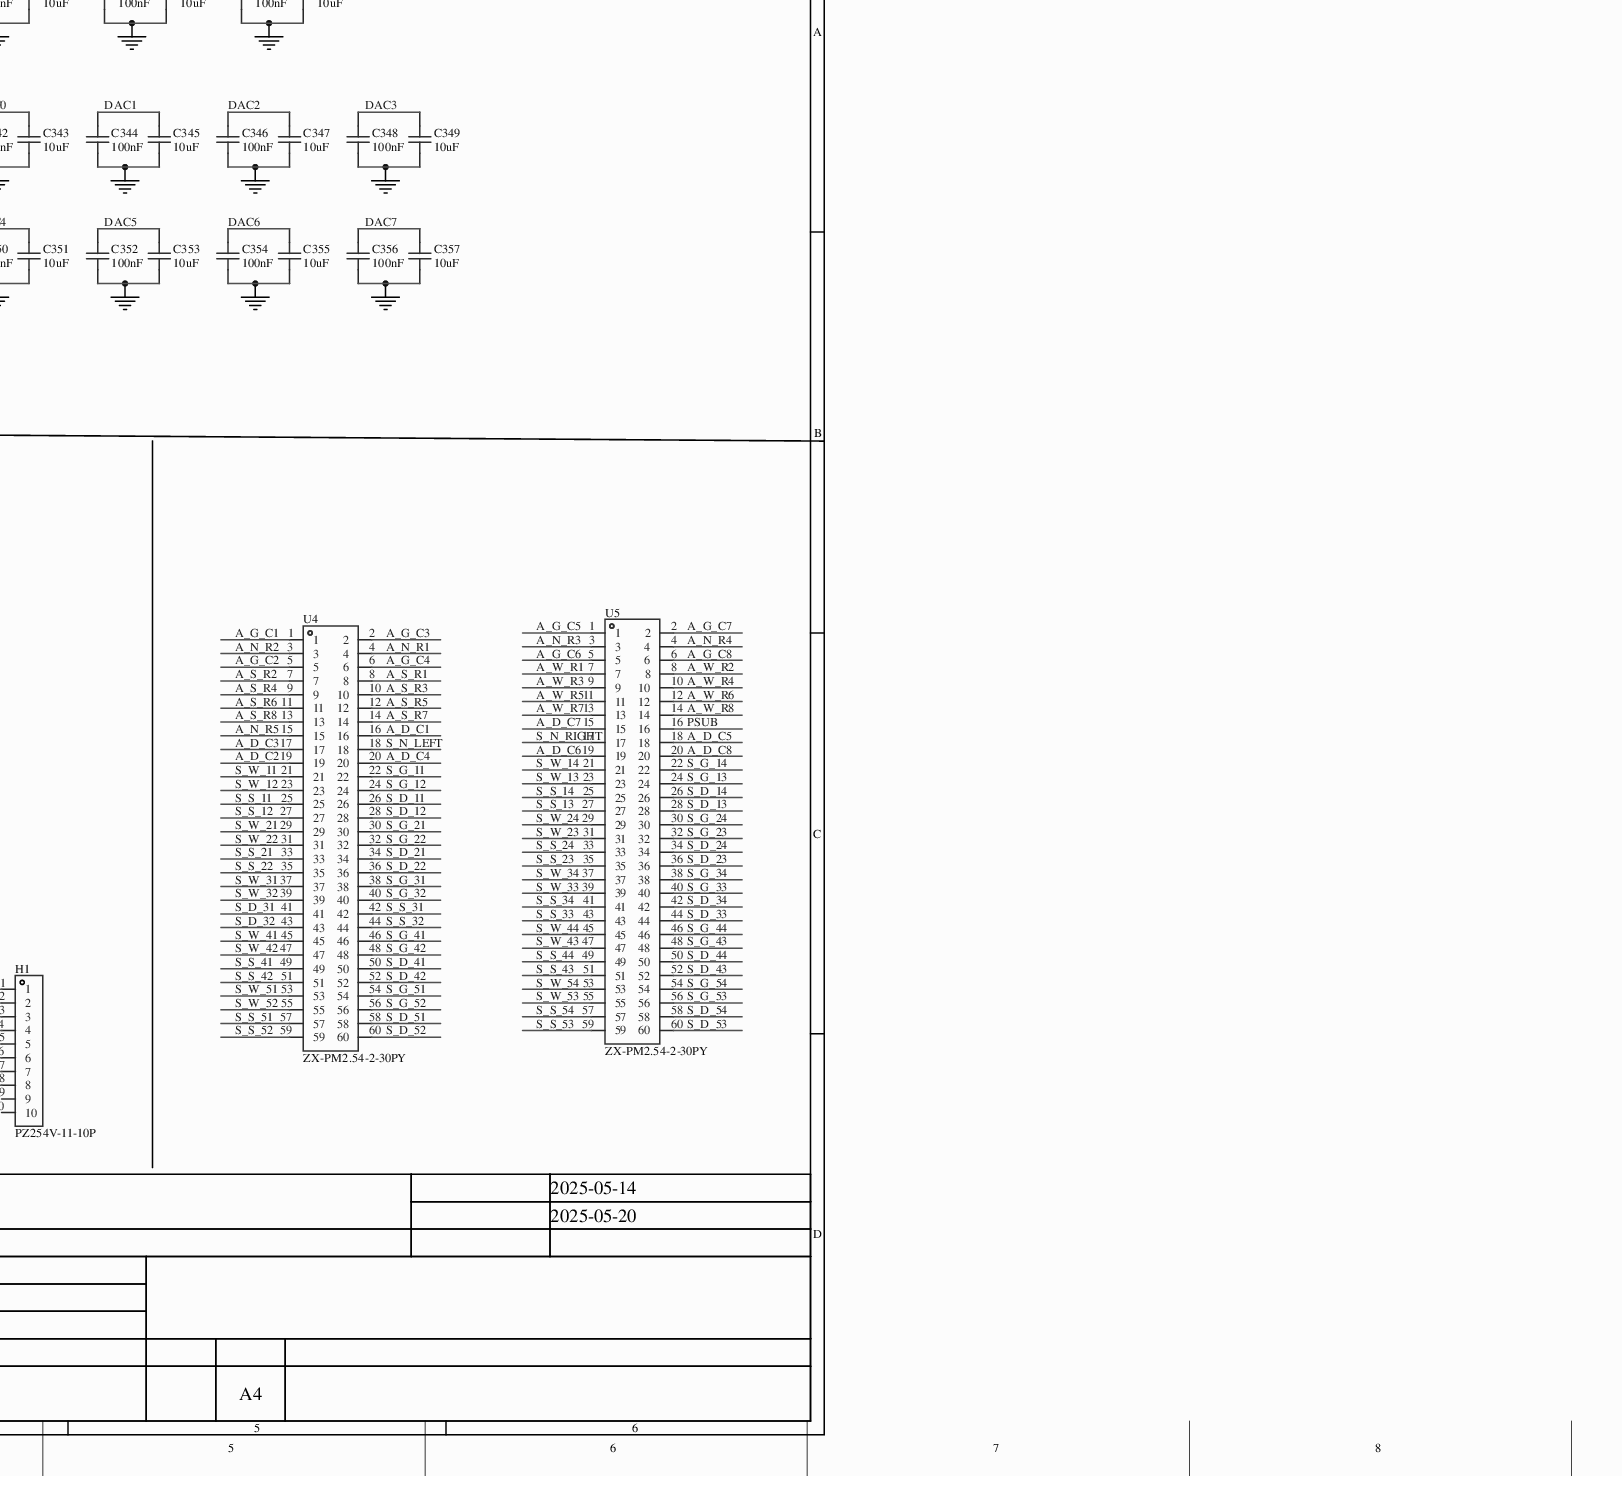
[diagram p0: MISC82799-2.schdoc, bottom column 2 of 4]
# Altium project MISC82799-9.PrjPCB (part 2 of 3)
## Sheet MISC82799-2.schdoc (continued)
### Library data of the parts (continued)
C330 = GRM21BR61H106KE43L: Add into BOM: yes; Voltage Rated: 50V; Temperature Coefficient: X5R; Symbol: 10uF; Device: GRM21BR61H106KE43L; Supplier Part: C440198; Manufacturer Part: GRM21BR61H106KE43L; Supplier Footprint: 0805; JLCPCB Part Class: Basic Part; Datasheet: https://example.com/upload/public/pdf/source/20230811/95AAE0C9AF55EDC31B7A4D8B733F534E.pdf; Supplier: LCSC; Convert to PCB: yes; Value: 10uF
C358 C359 = CL10A225KB8NNNC: Add into BOM: yes; Voltage Rated: 50V; Temperature Coefficient: X5R; Symbol: CL10A225KB8NNNC; Device: CL10A225KB8NNNC; Supplier Part: C913904; Manufacturer Part: CL10A225KB8NNNC; Supplier Footprint: 0603; Datasheet: https://example.com/upload/public/pdf/source/20160218/1457707763339.pdf; Supplier: LCSC; Convert to PCB: yes; Value: 2.2uF; Origin Footprint: C0603
C361-C363 = CL10A105KB8NNNC: Add into BOM: yes; Voltage Rated: 50V; Temperature Coefficient: X5R; Symbol: CL10A105KB8NNNC; Device: CL10A105KB8NNNC; Supplier Part: C15849; Manufacturer Part: CL10A105KB8NNNC; Supplier Footprint: 0603; Datasheet: https://example.com/upload/public/pdf/source/20160218/1457707763339.pdf; Supplier: LCSC; Convert to PCB: yes; Value: 1uF; Origin Footprint: C0603
D1 = VS-10BQ015HM3/5BT: Add into BOM: yes; Forward Voltage (Vf@If): 210mV@1A; Reverse Voltage (Vr): 15V; Rectified Current: 1A; Reverse Leakage Current (Ir): 500uA@15V; Symbol: VS-10BQ015HM3/5BT; Device: VS-10BQ015HM3/5BT; Supplier Part: C413465; Manufacturer Part: VS-10BQ015HM3/5BT; Supplier Footprint: DO-214AA(SMB); JLCPCB Part Class: Extended Part; Datasheet: https://example.com/upload/public/pdf/source/20190819/C413465_3D2B1A8C7366D4425AB887DF85498F89.pdf; Supplier: LCSC; Convert to PCB: yes
FPGAJ2 FPGAJ4 FPGAJ10 = 2.54-2*20: Add into BOM: yes; Holes Structure: 2x20P; Pitch: 2.54mm; Number of Holes: 40P; Current Rating (Max): 2.5A; Symbol: 2.54-2*20; Device: 2.54-2*20; Supplier Part: C2977589; Manufacturer Part: 2.54-2*20; JLCPCB Part Class: Extended Part; Datasheet: https://example.com/upload/public/pdf/source/20220328/834E302BE3C038BBC5C70F5E02589B1E.pdf; Supplier: LCSC; Convert to PCB: yes; Row Spacing: 2.54mm; Voltage Rating (Max): -; Insulation Height: 8.5mm
H1 = PZ254V-11-10P: Add into BOM: yes; Pin Structure: 1x10P; Pitch: 2.54mm; Symbol: PZ254V-11-10P; Device: PZ254V-11-10P; Supplier Part: C492409; Manufacturer Part: PZ254V-11-10P; JLCPCB Part Class: Extended Part; Datasheet: https://example.com/upload/public/pdf/source/20200309/C492409_129C9431BDD62EBBBD0A643B6AAB9FBD.pdf; Supplier: LCSC; Convert to PCB: yes; Row Spacing: -; Number of Pins: 10P; Current Rating: -; Voltage Rating (Max): -; Length of Mating Pin: 6mm; Insulation Height: 2.5mm; Length of End Connection Pin: 3mm; Contact Plating: -
H2 = PZ254-2-20-W-8.5_C2895000: Add into BOM: yes; Pin Structure: 2x20P; Pitch: 2.54mm; Current Rating (Max): 3A; Symbol: PZ254-2-20-W-8.5; Device: PZ254-2-20-W-8.5_C2895000; Supplier Part: C2895000; Manufacturer Part: PZ254-2-20-W-8.5; JLCPCB Part Class: Extended Part; Datasheet: https://example.com/upload/public/pdf/source/20230609/1B60364E488FD8696AA7206A46578DEA.pdf; Supplier: LCSC; Convert to PCB: yes; Row Spacing: 2.54mm; Number of Pins: 40P; Voltage Rating (Max): -; Length of Mating Pin: 6mm; Insulation Height: 2.5mm; Length of End Connection Pin: -; Contact Material: -
H3 = PZ254V-12-16P: Add into BOM: yes; Pin Structure: 2x8P; Pitch: 2.54mm; Symbol: PZ254V-12-16P; Device: PZ254V-12-16P; Supplier Part: C492425; Manufacturer Part: PZ254V-12-16P; JLCPCB Part Class: Extended Part; Datasheet: https://example.com/upload/public/pdf/source/20200309/C492425_0A00EE06259AD0A0AB9C88167BB69964.pdf; Supplier: LCSC; Convert to PCB: yes; Row Spacing: 2.54mm; Number of Pins: 16P; Current Rating: -; Voltage Rating (Max): -; Length of Mating Pin: 6mm; Insulation Height: 2.5mm; Length of End Connection Pin: 3mm; Contact Plating: -
H7 H9 = PZ254V-11-03P: Add into BOM: yes; Pin Structure: 1x3P; Pitch: 2.54mm; Current Rating: 3A; Voltage Rating (Max): 250V; Symbol: PZ254V-11-03P; Device: PZ254V-11-03P; Supplier Part: C2937625; Manufacturer Part: PZ254V-11-03P; Datasheet: https://example.com/upload/public/pdf/source/20200309/C492402_8335C3D49C4E4C618838D59BB1D024C1.pdf; Supplier: LCSC; Convert to PCB: yes; Row Spacing: -; Number of Pins: 3P; Length of Mating Pin: 6mm; Insulation Height: 2.5mm; Length of End Connection Pin: 3mm; Origin Footprint: HDR-TH_3P-P2.54-V-M
H8 = PZ254V-11-05P: Add into BOM: yes; Pin Structure: 1x5P; Pitch: 2.54mm; Symbol: PZ254V-11-05P; Device: PZ254V-11-05P; Supplier Part: C492404; Manufacturer Part: PZ254V-11-05P; Datasheet: https://example.com/upload/public/pdf/source/20200309/C492404_E51533260F8710EFF5D4617281164C1D.pdf; Supplier: LCSC; Convert to PCB: yes; Row Spacing: -; Number of Pins: 5P; Current Rating: -; Voltage Rating (Max): -; Length of Mating Pin: 6mm; Insulation Height: 2.5mm; Length of End Connection Pin: 3mm; Contact Plating: -; Origin Footprint: HDR-TH_5P-P2.54-V-M
L3 = PCAQ7060MW-301: Add into BOM: yes; Number of Lines: 2; Voltage Withstand: 125V; Current Rating: 5A; Symbol: PCAQ7060MW-301; Device: PCAQ7060MW-301; Supplier Part: C2916896; Manufacturer Part: PCAQ7060MW-301; Supplier Footprint: SMD,7x6x3.8mm; Datasheet: https://example.com/upload/public/pdf/source/20220923/2764902BE544E236930A8CC0DC83284B.pdf; Supplier: LCSC; Convert to PCB: yes; Inductance @ Frequency: -; Voltage Rating - DC: 125V; Voltage Rating (AC): -; Origin Footprint: FILTER-SMD_4P-L7.0-W6.0-BL
LED1 = NCD0805G1: Add into BOM: yes; Forward Voltage (VF): 2.5V~3.6V; Power Dissipation: 72mW; Forward Current: 5mA; Dominant Wavelength: 525nm~537.5nm; Luminous Intensity: 180mcd~400mcd; Symbol: NCD0805G1; Device: NCD0805G1; LCSC Part Name: NCD0805G1; Supplier Part: C84260; Manufacturer Part: NCD0805G1; Supplier Footprint: 0805; JLCPCB Part Class: Extended Part; Datasheet: https://example.com/upload/public/pdf/source/20200820/C84260_AFC7BF57C6FBA034D182BB8D10A67EFE.pdf; Supplier: LCSC; Convert to PCB: yes
R25 = 0603WAF1004T5E: Add into BOM: yes; Power(Watts): 100mW; Overload Voltage (Max): 75V; Symbol: 0603WAF1004T5E; Device: 0603WAF1004T5E; Supplier Part: C22935; Manufacturer Part: 0603WAF1004T5E; Supplier Footprint: 0603; JLCPCB Part Class: Basic Part; Datasheet: https://example.com/upload/public/pdf/source/20200306/C422600_1E6D84923E4A46A82E41ADD87F860B5C.pdf; Supplier: LCSC; Convert to PCB: yes
R27 = RT0603BRD07681RL: Add into BOM: yes; Power(Watts): 100mW; Overload Voltage (Max): 75V; Symbol: RT0603BRD07681RL; Device: RT0603BRD07681RL; Supplier Part: C705792; Manufacturer Part: RT0603BRD07681RL; Supplier Footprint: 0603; JLCPCB Part Class: Extended Part; Datasheet: https://example.com/upload/public/pdf/source/20200720/C705792_EDF314EE001EB4AE666F730223633204.pdf; Supplier: LCSC; Convert to PCB: yes
R28 = 0603WAF1001T5E: Add into BOM: yes; Power(Watts): 100mW; Overload Voltage (Max): 75V; Symbol: 0603WAF1001T5E; Device: 0603WAF1001T5E; Supplier Part: C21190; Manufacturer Part: 0603WAF1001T5E; Supplier Footprint: 0603; JLCPCB Part Class: Basic Part; Datasheet: https://example.com/upload/public/pdf/source/20200306/C422600_1E6D84923E4A46A82E41ADD87F860B5C.pdf; Supplier: LCSC; Convert to PCB: yes
R165 = 0603WAF4533T5E: Add into BOM: yes; Power(Watts): 100mW; Overload Voltage (Max): 75V; Symbol: 0603WAF4533T5E; Device: 0603WAF4533T5E; Supplier Part: C25818; Manufacturer Part: 0603WAF4533T5E; Supplier Footprint: 0603; JLCPCB Part Class: Extended Part; Datasheet: https://example.com/upload/public/pdf/source/20200306/C422600_1E6D84923E4A46A82E41ADD87F860B5C.pdf; Supplier: LCSC; Convert to PCB: yes
R166 = AR03BTC5002A: Add into BOM: yes; Power(Watts): 62.5mW; Symbol: AR03BTC5002A; Device: AR03BTC5002A; Supplier Part: C304067; Manufacturer Part: AR03BTC5002A; Supplier Footprint: 0603; JLCPCB Part Class: Extended Part; Datasheet: https://example.com/upload/public/pdf/source/20180929/C304149_5A5914DE4BA6462262A23A17FA3D8526.pdf; Supplier: LCSC; Convert to PCB: yes
R167 = 0603WAF2490T5E: Add into BOM: yes; Power(Watts): 100mW; Overload Voltage (Max): 75V; Symbol: 0603WAF2490T5E; Device: 0603WAF2490T5E; Supplier Part: C22919; Manufacturer Part: 0603WAF2490T5E; Supplier Footprint: 0603; JLCPCB Part Class: Extended Part; Datasheet: https://example.com/upload/public/pdf/source/20200306/C422600_1E6D84923E4A46A82E41ADD87F860B5C.pdf; Supplier: LCSC; Convert to PCB: yes
R168 = 0603WAF2003T5E: Add into BOM: yes; Power(Watts): 100mW; Overload Voltage (Max): 75V; Symbol: 0603WAF2003T5E; Device: 0603WAF2003T5E; Supplier Part: C25811; Manufacturer Part: 0603WAF2003T5E; Supplier Footprint: 0603; JLCPCB Part Class: Basic Part; Datasheet: https://example.com/upload/public/pdf/source/20200306/C422600_1E6D84923E4A46A82E41ADD87F860B5C.pdf; Supplier: LCSC; Convert to PCB: yes
R169 = ERJ3RED3573V: Add into BOM: yes; Power(Watts): 100mW; Voltage-Supply(Max): 100V; Symbol: ERJ3RED3573V; Device: ERJ3RED3573V; Supplier Part: C278649; Manufacturer Part: ERJ3RED3573V; Supplier Footprint: 0603; Datasheet: https://example.com/upload/public/pdf/source/20181114/C278649_3EAAB526D833AC096AA76B5DF119202B.pdf; Supplier: LCSC; Convert to PCB: yes; Origin Footprint: R0603
R170 = 0603WAF7502T5E: Add into BOM: yes; Power(Watts): 100mW; Overload Voltage (Max): 75V; Symbol: 0603WAF7502T5E; Device: 0603WAF7502T5E; Supplier Part: C23242; Manufacturer Part: 0603WAF7502T5E; Supplier Footprint: 0603; Datasheet: https://example.com/upload/public/pdf/source/20200306/C422600_1E6D84923E4A46A82E41ADD87F860B5C.pdf; Supplier: LCSC; Convert to PCB: yes; Origin Footprint: R0603
SW1 = K3-1204D: Add into BOM: yes; Switch Length: 10mm; Switch Width: 2.5mm; Switch Height: 6mm; Current Rating (AC): 5A; Voltage Rating (AC): 120V; Symbol: K3-1204D; Device: K3-1204D; Supplier Part: C145861; Manufacturer Part: K3-1204D; JLCPCB Part Class: Extended Part; Datasheet: https://example.com/upload/public/pdf/source/20210810/A7BCE8A3AE6875067403B729968221B7.pdf; Supplier: LCSC; Convert to PCB: yes; Actuator Style: -; Voltage Rating (DC): -
TP13 = 5V: Add into BOM: yes; Symbol: 5V; Device: 5V; Convert to PCB: yes; Origin Footprint: Test-Point-0.5mm; Design Item ID: Test-Point
TP14 = 3P3V: Add into BOM: yes; Symbol: 3P3V; Device: 3P3V; Convert to PCB: yes; Origin Footprint: Test-Point-0.5mm; Design Item ID: Test-Point
U4 U5 = ZX-PM2.54-2-30PY: Add into BOM: yes; Holes Structure: 2x30P; Pitch: 2.54mm; Number of Holes: 60P; Voltage Rating (Max): 1kV; Symbol: ZX-PM2.54-2-30PY; Device: ZX-PM2.54-2-30PY; Supplier Part: C7499356; Manufacturer Part: ZX-PM2.54-2-30PY; JLCPCB Part Class: Extended Part; Datasheet: https://example.com/upload/public/pdf/source/20231122/23E1107B34356833C267F6B6E856DE02.pdf; Supplier: LCSC; Convert to PCB: yes; Row Spacing: 2.54mm; Current Rating (Max): -; Insulation Height: 8.5mm; Contact Material: -
U39 = HX DC007B-2.5: Add into BOM: yes; Inside Contact Diameter: 2.5mm; Outside Contact Diameter: 6.4mm; Current Rating (Max): 7A; Voltage Rating (Max): 20V; Symbol: HX DC007B-2.5; Device: HX DC007B-2.5; Supplier Part: C19189083; Manufacturer Part: HX DC007B-2.5; JLCPCB Part Class: Extended Part; Datasheet: https://example.com/upload/public/pdf/source/20231103/814B3421283469BAAEFFF9B7A53EC0CB.pdf; Supplier: LCSC; Convert to PCB: yes
U40 = SMAJ12CA: Manufacturer: KUU; Add into BOM: yes; Reverse Stand-Off Voltage (Vrwm): 12V; Maximum Clamping Voltage: 19.9V; Peak Pulse Current (Ipp)@10/1000us: 20.1A; Peak Pulse Power Dissipation (Ppp)@10/1000us: 400W; Breakdown Voltage: 13.3V; Reverse Leakage Current (Ir): 1uA; Symbol: SMAJ12CA; Device: SMAJ12CA; Supplier Part: C2985628; Manufacturer Part: SMAJ12CA; Supplier Footprint: SMA; Datasheet: https://example.com/upload/public/pdf/source/20211202/BA5FA378886C9E49EA844EF3397415D6.pdf; Supplier: LCSC; Convert to PCB: yes; Type: TVS; Origin Footprint: SMA_L4.3-W2.7-LS5.1-BI; Design Item ID: SMAJ12CA
U41 = TPS259472ARPWR: Add into BOM: yes; Voltage Rating: 2.7V~23V; Symbol: TPS259472ARPWR; Device: TPS259472ARPWR; LCSC Part Name: TPS259472ARPWR; Supplier Part: C3662789; Manufacturer Part: TPS259472ARPWR; Supplier Footprint: VQFN-10-HR(2x2); JLCPCB Part Class: Extended Part; Supplier: LCSC; Convert to PCB: yes
U42 U43 = CL21A226KOQNNNE: Add into BOM: yes; Voltage Rated: 16V; Temperature Coefficient: X5R; Symbol: 22uF; Device: CL21A226KOQNNNE; Supplier Part: C296720; Manufacturer Part: CL21A226KOQNNNE; Supplier Footprint: 0805; JLCPCB Part Class: Extended Part; Datasheet: https://example.com/upload/public/pdf/source/20160218/1457707763339.pdf; Supplier: LCSC; Convert to PCB: yes; Value: 22uF
U91 = LT3045IDD#PBF: Add into BOM: yes; Maximum Input Voltage: 20V; Output Voltage: 0V~15V; Output Current: 500mA; Dropout Voltage: 450mV@(500mA); standby current: 20uA; Number of Outputs: 1; Symbol: LT3045IDD#PBF; Device: LT3045IDD#PBF; Supplier Part: C580013; Manufacturer Part: LT3045IDD#PBF; Supplier Footprint: DFN-10-EP(3x3); JLCPCB Part Class: Extended Part; Datasheet: https://example.com/upload/public/pdf/source/20200416/C514420_E440C492D6C74EAE6AB301243586F696.pdf; Supplier: LCSC; Convert to PCB: yes
U96 = DAC80508ZRTER: Add into BOM: yes; Interface: SPI; Supply Voltage: 1.7V~5.5V; Settling Time: 5us; Symbol: DAC80508ZRTER; Device: DAC80508ZRTER; LCSC Part Name: DAC80508ZRTER; Supplier Part: C2679499; Manufacturer Part: DAC80508ZRTER; Supplier Footprint: WQFN-16-EP(3x3); JLCPCB Part Class: Extended Part; Supplier: LCSC; Convert to PCB: yes
U143 = TPS60403DBVR: Add into BOM: yes; Symbol: TPS60403DBVR; Device: TPS60403DBVR; LCSC Part Name: TPS60403DBVR; Supplier Part: C11338; Manufacturer Part: TPS60403DBVR; Supplier Footprint: SOT-23-5; Supplier: LCSC; Convert to PCB: yes; Origin Footprint: SOT-23-5_L3.0-W1.7-P0.95-LS2.8-BR
U144 = TPS72301DBVR: Add into BOM: yes; Maximum Input Voltage: 10V; Output Voltage: 1.2V~10V; MAX Output Current: 200mA; Power Supply Rejection Ratio (PSRR): 65dB; Dropout Voltage: 500mV@(200mA); standby current: 200uA; Number of Outputs: 1; Symbol: TPS72301DBVR; Device: TPS72301DBVR; Supplier Part: C34678; Manufacturer Part: TPS72301DBVR; Supplier Footprint: SOT-23-5; Supplier: LCSC; Convert to PCB: yes; Origin Footprint: SOT-23-5_L3.0-W1.7-P0.95-LS2.8-BR
VR11 VR12 = 3224W-1-503E: Manufacturer: BOURNS; Resistance: 50K; Add into BOM: yes; Power(Watts): 250mW; Turns: 12; Symbol: 3224W-1-503E; Device: 3224W-1-503E; Supplier: LCSC; Manufacturer Part: 3224W-1-503E; Supplier Part: C48484; Supplier Footprint: SMD; Datasheet: https://example.com/upload/public/pdf/source/20160830/1472551532733.pdf; Convert to PCB: yes; Origin Footprint: RES-ADJ-SMD_3224W
  VR11: Design Item ID: 3224W-1-503E

## Sheet MISC82799-4.schdoc
size 309 x 223 mm; Name: MISC82799; @Page No: 2; @Page Count: 2; @Schematic Name: MISC82799; @Project Name: MISC82799; @Board Name: MISC82799; @Update Date: 2025-05-26; @Create Time: 16:47:34; @Update Time: 16:47:50; @Create Date: 2025-05-26
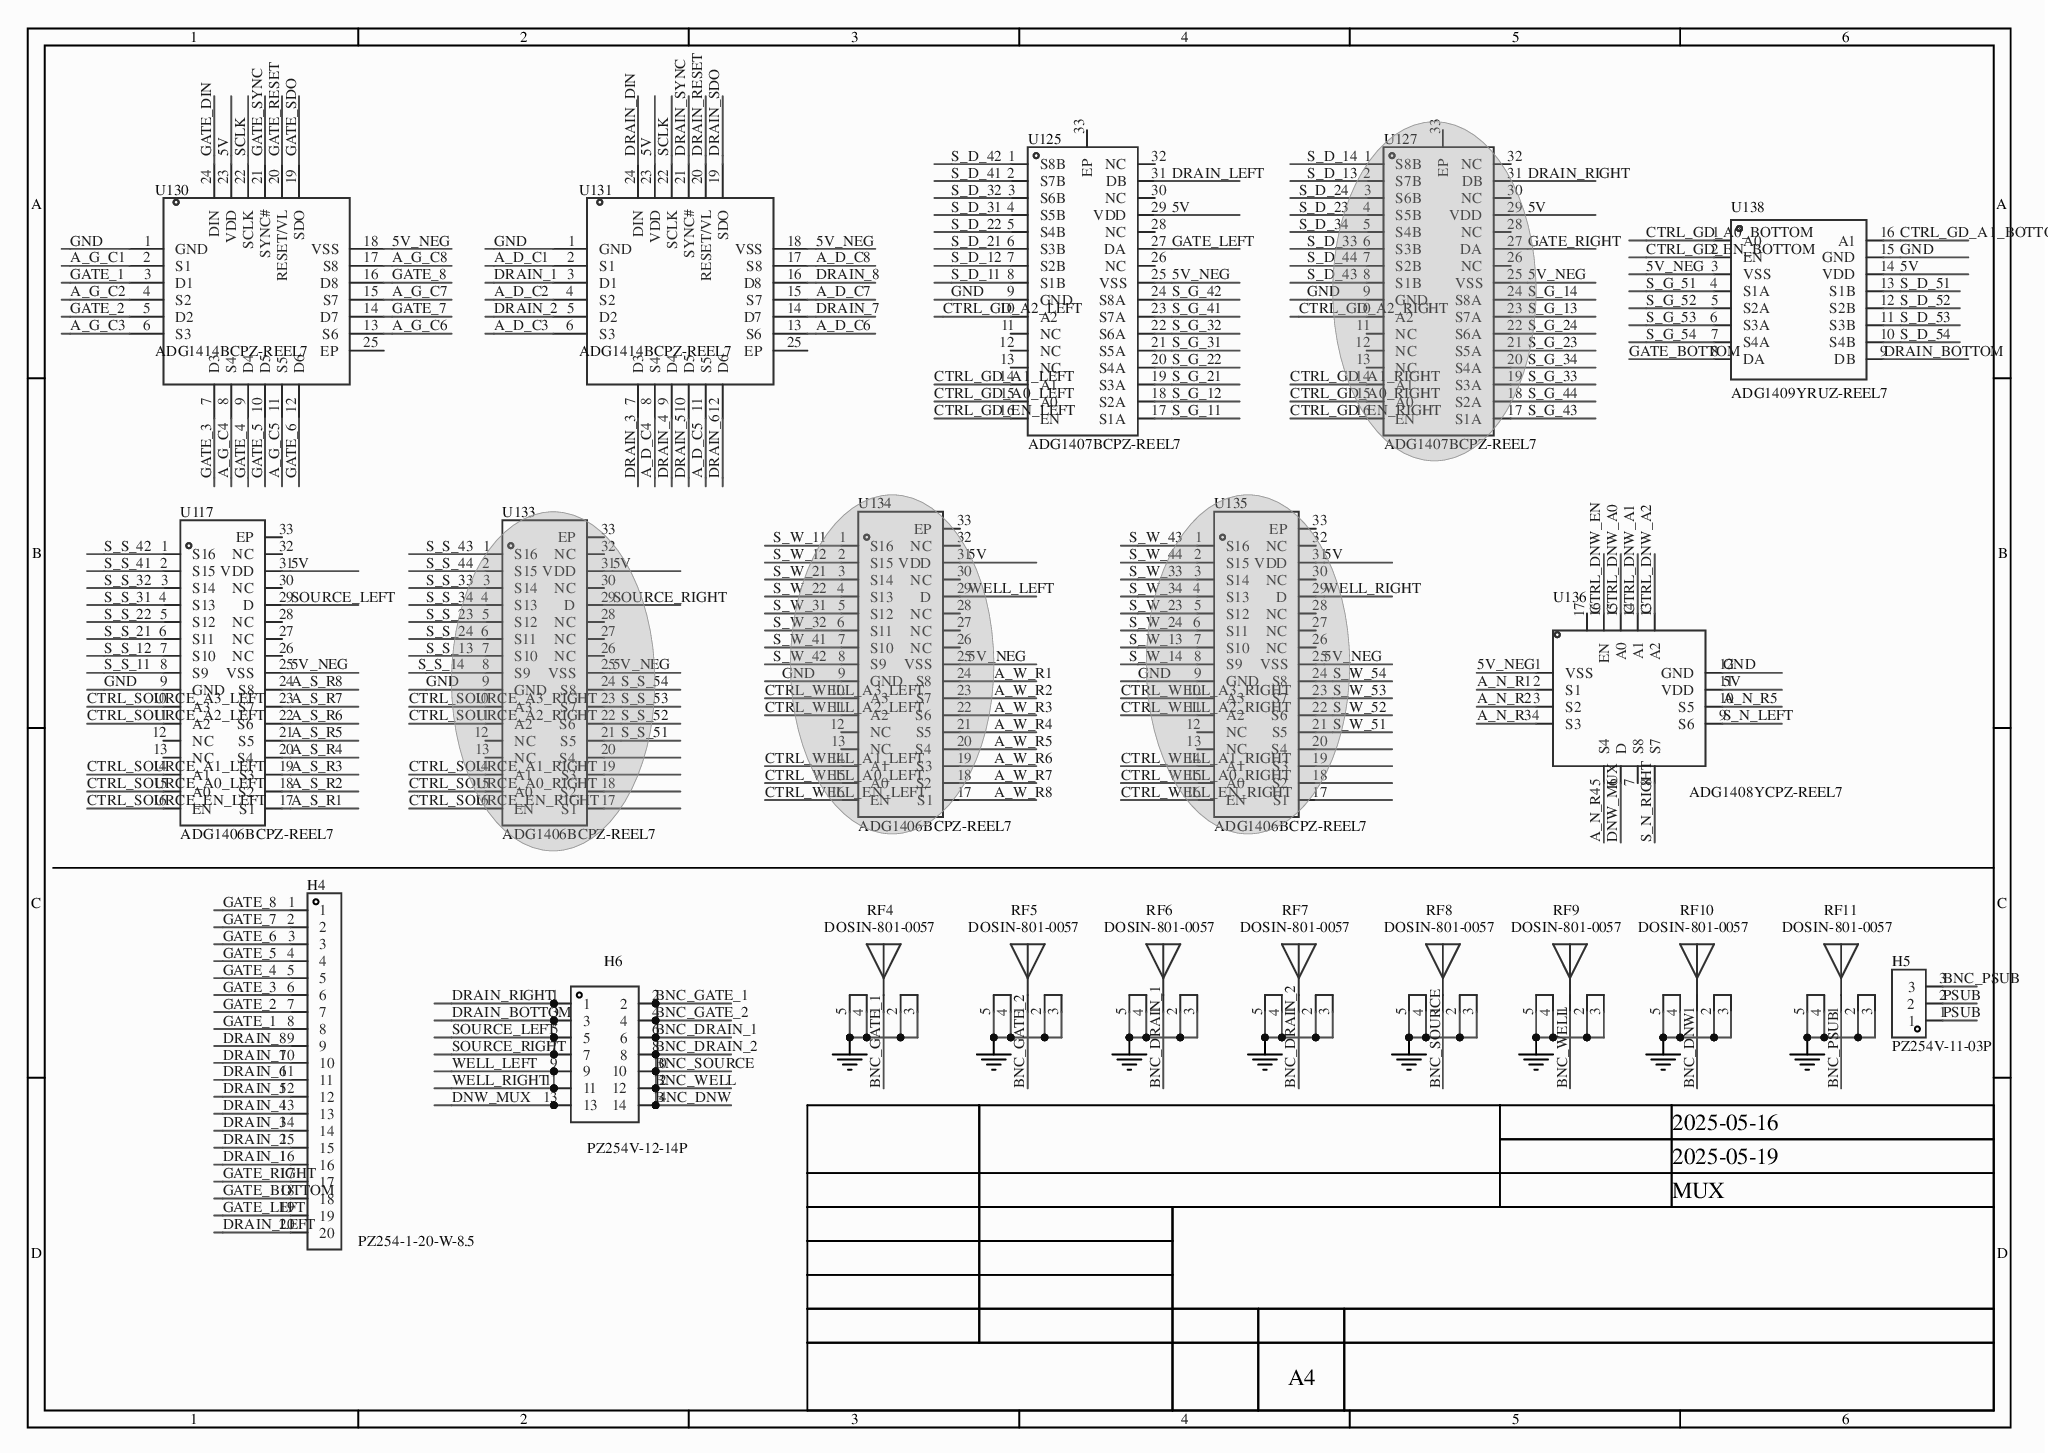
[diagram p1: MISC82799-4.schdoc]

### Parts
H4  PZ254-1-20-W-8.5  [HDR-TH_20P-P2.54-V-M-1]
H5  PZ254V-11-03P  [HDR-TH_3P-P2.54-V-M]
H6  PZ254V-12-14P  [HDR-TH_14P-P2.54-V-M-R2-C7-S2.54]
RF4  DOSIN-801-0057  [ANT-TH_DOSIN-801-0057]
RF5  DOSIN-801-0057  [ANT-TH_DOSIN-801-0057]
RF6  DOSIN-801-0057  [ANT-TH_DOSIN-801-0057]
RF7  DOSIN-801-0057  [ANT-TH_DOSIN-801-0057]
RF8  DOSIN-801-0057  [ANT-TH_DOSIN-801-0057]
RF9  DOSIN-801-0057  [ANT-TH_DOSIN-801-0057]
RF10  DOSIN-801-0057  [ANT-TH_DOSIN-801-0057]
RF11  DOSIN-801-0057  [ANT-TH_DOSIN-801-0057]
U117  ADG1406BCPZ-REEL7  [LFCSP-32_L5.0-W5.0-P0.50-TL-EP3.1]
U125  ADG1407BCPZ-REEL7  [LFCSP-32_L5.0-W5.0-P0.50-BL-EP3.1]
U127  ADG1407BCPZ-REEL7  [LFCSP-32_L5.0-W5.0-P0.50-BL-EP3.1]
U130  ADG1414BCPZ-REEL7  [LFCSP-24_L4.0-W4.0-P0.50-BL-EP]
U131  ADG1414BCPZ-REEL7  [LFCSP-24_L4.0-W4.0-P0.50-BL-EP]
U133  ADG1406BCPZ-REEL7  [LFCSP-32_L5.0-W5.0-P0.50-TL-EP3.1]
U134  ADG1406BCPZ-REEL7  [LFCSP-32_L5.0-W5.0-P0.50-TL-EP3.1]
U135  ADG1406BCPZ-REEL7  [LFCSP-32_L5.0-W5.0-P0.50-TL-EP3.1]
U136  ADG1408YCPZ-REEL7  [LFCSP-16_L4.0-W4.0-P0.65-BL-EP]
U138  ADG1409YRUZ-REEL7  [TSSOP-16_L5.0-W4.4-P0.65-LS6.4-BL]

### Nets
GND: RF4.2 RF4.3 RF4.4 RF4.5 RF5.2 RF5.3 RF5.4 RF5.5 RF6.2 RF6.3 RF6.4 RF6.5 RF7.2 RF7.3 RF7.4 RF7.5 RF8.2 RF8.3 RF8.4 RF8.5 RF9.2 RF9.3 RF9.4 RF9.5 RF10.2 RF10.3 RF10.4 RF10.5 RF11.2 RF11.3 RF11.4 RF11.5 U117.9(GND) U125.9(GND) U127.9(GND) U130.1(GND) U131.1(GND) U133.9(GND) U134.9(GND) U135.9(GND) U136.12(GND) U138.15(GND)
5V: U117.31(VDD) U125.29(VDD) U127.29(VDD) U130.23(VDD) U131.23(VDD) U133.31(VDD) U134.31(VDD) U135.31(VDD) U136.11(VDD) U138.14(VDD)
5V_NEG: U117.25(VSS) U125.25(VSS) U127.25(VSS) U130.18(VSS) U131.18(VSS) U133.25(VSS) U134.25(VSS) U135.25(VSS) U136.1(VSS) U138.3(VSS)
A_D_C1: U131.2(S1)
A_D_C2: U131.4(S2)
A_D_C3: U131.6(S3)
A_D_C4: U131.8(S4)
A_D_C5: U131.11(S5)
A_D_C6: U131.13(S6)
A_D_C7: U131.15(S7)
A_D_C8: U131.17(S8)
A_G_C1: U130.2(S1)
A_G_C2: U130.4(S2)
A_G_C3: U130.6(S3)
A_G_C4: U130.8(S4)
A_G_C5: U130.11(S5)
A_G_C6: U130.13(S6)
A_G_C7: U130.15(S7)
A_G_C8: U130.17(S8)
A_N_R1: U136.2(S1)
A_N_R2: U136.3(S2)
A_N_R3: U136.4(S3)
A_N_R4: U136.5(S4)
A_N_R5: U136.10(S5)
A_S_R1: U117.17(S1)
A_S_R2: U117.18(S2)
A_S_R3: U117.19(S3)
A_S_R4: U117.20(S4)
A_S_R5: U117.21(S5)
A_S_R6: U117.22(S6)
A_S_R7: U117.23(S7)
A_S_R8: U117.24(S8)
A_W_R1: U134.24(S8)
A_W_R2: U134.23(S7)
A_W_R3: U134.22(S6)
A_W_R4: U134.21(S5)
A_W_R5: U134.20(S4)
A_W_R6: U134.19(S3)
A_W_R7: U134.18(S2)
A_W_R8: U134.17(S1)
BNC_DNW: H6.14 RF10.1
BNC_DRAIN_1: H6.6 RF6.1
BNC_DRAIN_2: H6.8 RF7.1
BNC_GATE_1: H6.2 RF4.1
BNC_GATE_2: H6.4 RF5.1
BNC_PSUB: H5.3 RF11.1
BNC_SOURCE: H6.10 RF8.1
BNC_WELL: H6.12 RF9.1
CTRL_DNW_A0: U136.15(A0)
CTRL_DNW_A1: U136.14(A1)
CTRL_DNW_A2: U136.13(A2)
CTRL_DNW_EN: U136.16(EN)
CTRL_GD_A0_BOTTOM: U138.1(A0)
CTRL_GD_A0_LEFT: U125.15(A0)
CTRL_GD_A0_RIGHT: U127.15(A0)
CTRL_GD_A1_BOTTOM: U138.16(A1)
CTRL_GD_A1_LEFT: U125.14(A1)
CTRL_GD_A1_RIGHT: U127.14(A1)
CTRL_GD_A2_LEFT: U125.10(A2)
CTRL_GD_A2_RIGHT: U127.10(A2)
CTRL_GD_EN_BOTTOM: U138.2(EN)
CTRL_GD_EN_LEFT: U125.16(EN)
CTRL_GD_EN_RIGHT: U127.16(EN)
CTRL_SOURCE_A0_LEFT: U117.15(A0)
CTRL_SOURCE_A0_RIGHT: U133.15(A0)
CTRL_SOURCE_A1_LEFT: U117.14(A1)
CTRL_SOURCE_A1_RIGHT: U133.14(A1)
CTRL_SOURCE_A2_LEFT: U117.11(A2)
CTRL_SOURCE_A2_RIGHT: U133.11(A2)
CTRL_SOURCE_A3_LEFT: U117.10(A3)
CTRL_SOURCE_A3_RIGHT: U133.10(A3)
CTRL_SOURCE_EN_LEFT: U117.16(EN)
CTRL_SOURCE_EN_RIGHT: U133.16(EN)
CTRL_WELL_A0_LEFT: U134.15(A0)
CTRL_WELL_A0_RIGHT: U135.15(A0)
CTRL_WELL_A1_LEFT: U134.14(A1)
CTRL_WELL_A1_RIGHT: U135.14(A1)
CTRL_WELL_A2_LEFT: U134.11(A2)
CTRL_WELL_A2_RIGHT: U135.11(A2)
CTRL_WELL_A3_LEFT: U134.10(A3)
CTRL_WELL_A3_RIGHT: U135.10(A3)
CTRL_WELL_EN_LEFT: U134.16(EN)
CTRL_WELL_EN_RIGHT: U135.16(EN)
DNW_MUX: H6.13 U136.6(D)
DRAIN_1: H4.16 U131.3(D1)
DRAIN_2: H4.15 U131.5(D2)
DRAIN_3: H4.14 U131.7(D3)
DRAIN_4: H4.13 U131.9(D4)
DRAIN_5: H4.12 U131.10(D5)
DRAIN_6: H4.11 U131.12(D6)
DRAIN_7: H4.10 U131.14(D7)
DRAIN_8: H4.9 U131.16(D8)
DRAIN_BOTTOM: H6.3 U138.9(DB)
DRAIN_DIN: U131.24(DIN)
DRAIN_LEFT: H4.20 U125.31(DB)
DRAIN_RESET: U131.20(RESET/VL)
DRAIN_RIGHT: H6.1 U127.31(DB)
DRAIN_SDO: U131.19(SDO)
DRAIN_SYNC: U131.21(SYNC#)
GATE_1: H4.8 U130.3(D1)
GATE_2: H4.7 U130.5(D2)
GATE_3: H4.6 U130.7(D3)
GATE_4: H4.5 U130.9(D4)
GATE_5: H4.4 U130.10(D5)
GATE_6: H4.3 U130.12(D6)
GATE_7: H4.2 U130.14(D7)
GATE_8: H4.1 U130.16(D8)
GATE_BOTTOM: H4.18 U138.8(DA)
GATE_DIN: U130.24(DIN)
GATE_LEFT: H4.19 U125.27(DA)
GATE_RESET: U130.20(RESET/VL)
GATE_RIGHT: H4.17 U127.27(DA)
GATE_SDO: U130.19(SDO)
GATE_SYNC: U130.21(SYNC#)
PSUB: H5.1 H5.2
S_D_11: U125.8(S1B)
S_D_12: U125.7(S2B)
S_D_13: U127.2(S7B)
S_D_14: U127.1(S8B)
S_D_21: U125.6(S3B)
S_D_22: U125.5(S4B)
S_D_23: U127.4(S5B)
S_D_24: U127.3(S6B)
S_D_31: U125.4(S5B)
S_D_32: U125.3(S6B)
S_D_33: U127.6(S3B)
S_D_34: U127.5(S4B)
S_D_41: U125.2(S7B)
S_D_42: U125.1(S8B)
S_D_43: U127.8(S1B)
S_D_44: U127.7(S2B)
S_D_51: U138.13(S1B)
S_D_52: U138.12(S2B)
S_D_53: U138.11(S3B)
S_D_54: U138.10(S4B)
S_G_11: U125.17(S1A)
S_G_12: U125.18(S2A)
S_G_13: U127.23(S7A)
S_G_14: U127.24(S8A)
S_G_21: U125.19(S3A)
S_G_22: U125.20(S4A)
S_G_23: U127.21(S5A)
S_G_24: U127.22(S6A)
S_G_31: U125.21(S5A)
S_G_32: U125.22(S6A)
S_G_33: U127.19(S3A)
S_G_34: U127.20(S4A)
S_G_41: U125.23(S7A)
S_G_42: U125.24(S8A)
S_G_43: U127.17(S1A)
S_G_44: U127.18(S2A)
S_G_51: U138.4(S1A)
S_G_52: U138.5(S2A)
S_G_53: U138.6(S3A)
S_G_54: U138.7(S4A)
S_N_LEFT: U136.9(S6)
S_N_RIGHT: U136.8(S7)
S_S_11: U117.8(S9)
S_S_12: U117.7(S10)
S_S_13: U133.7(S10)
S_S_14: U133.8(S9)
S_S_21: U117.6(S11)
S_S_22: U117.5(S12)
S_S_23: U133.5(S12)
S_S_24: U133.6(S11)
S_S_31: U117.4(S13)
S_S_32: U117.3(S14)
S_S_33: U133.3(S14)
S_S_34: U133.4(S13)
S_S_41: U117.2(S15)
S_S_42: U117.1(S16)
S_S_43: U133.1(S16)
S_S_44: U133.2(S15)
S_S_51: U133.21(S5)
S_S_52: U133.22(S6)
S_S_53: U133.23(S7)
S_S_54: U133.24(S8)
S_W_11: U134.1(S16)
S_W_12: U134.2(S15)
S_W_13: U135.7(S10)
S_W_14: U135.8(S9)
S_W_21: U134.3(S14)
S_W_22: U134.4(S13)
S_W_23: U135.5(S12)
S_W_24: U135.6(S11)
S_W_31: U134.5(S12)
S_W_32: U134.6(S11)
S_W_33: U135.3(S14)
S_W_34: U135.4(S13)
S_W_41: U134.7(S10)
S_W_42: U134.8(S9)
S_W_43: U135.1(S16)
S_W_44: U135.2(S15)
S_W_51: U135.21(S5)
S_W_52: U135.22(S6)
S_W_53: U135.23(S7)
S_W_54: U135.24(S8)
SCLK: U130.22(SCLK) U131.22(SCLK)
SOURCE_LEFT: H6.5 U117.29(D)
SOURCE_RIGHT: H6.7 U133.29(D)
WELL_LEFT: H6.9 U134.29(D)
WELL_RIGHT: H6.11 U135.29(D)

Not connected (* = marked no-connect by the designer): U117 12(NC) 13(NC) 26(NC) 27(NC) 28(NC) 30(NC) 32(NC) 33(EP); U125 11(NC) 12(NC) 13(NC) 26(NC) 28(NC) 30(NC) 32(NC) 33(EP); U127 11(NC) 12(NC) 13(NC) 26(NC) 28(NC) 30(NC) 32(NC) 33(EP); U130 25(EP); U131 25(EP); U133 12(NC) 13(NC) 17(S1) 18(S2) 19(S3) 20(S4) 26(NC) 27(NC) 28(NC) 30(NC) 32(NC) 33(EP); U134 12(NC) 13(NC) 26(NC) 27(NC) 28(NC) 30(NC) 32(NC) 33(EP); U135 12(NC) 13(NC) 17(S1) 18(S2) 19(S3) 20(S4) 26(NC) 27(NC) 28(NC) 30(NC) 32(NC) 33(EP); U136 7(S8) 17

### Notes on the sheet
- 1
- 2
- 3
- 4
- 5
- 6
- A
- B
- C
- 2025-05-16
- 2025-05-19
- D
- MUX
- A4

### Library data of the parts
H4 = PZ254-1-20-W-8.5: Add into BOM: yes; Pin Structure: 1x20P; Pitch: 2.54mm; Current Rating: 3A; Symbol: PZ254-1-20-W-8.5; Device: PZ254-1-20-W-8.5; Supplier Part: C2894962; Manufacturer Part: PZ254-1-20-W-8.5; JLCPCB Part Class: Extended Part; Datasheet: https://example.com/upload/public/pdf/source/20230609/872AF364EDF8DB2CAF0930EAB94ECB6E.pdf; Supplier: LCSC; Convert to PCB: yes; Row Spacing: -; Number of Pins: 20P; Voltage Rating (Max): -; Length of Mating Pin: 6mm; Insulation Height: 2.5mm; Length of End Connection Pin: -; Contact Material: -
H5 = PZ254V-11-03P: as H7 on sheet MISC82799-2; Symbol: PZ254V-11-03P; Device: PZ254V-11-03P; Supplier Part: C2937625; Manufacturer Part: PZ254V-11-03P; Datasheet: https://example.com/upload/public/pdf/source/20200309/C492402_8335C3D49C4E4C618838D59BB1D024C1.pdf; Supplier: LCSC; Convert to PCB: yes; Row Spacing: -; Number of Pins: 3P; Length of Mating Pin: 6mm; Insulation Height: 2.5mm; Length of End Connection Pin: 3mm; Origin Footprint: HDR-TH_3P-P2.54-V-M
H6 = PZ254V-12-14P: Add into BOM: yes; Pin Structure: 2x7P; Pitch: 2.54mm; Symbol: PZ254V-12-14P; Device: PZ254V-12-14P; Supplier Part: C492424; Manufacturer Part: PZ254V-12-14P; JLCPCB Part Class: Extended Part; Datasheet: https://example.com/upload/public/pdf/source/20200309/C492424_D71F2B7B4151908BA6AE7E1F567EA536.pdf; Supplier: LCSC; Convert to PCB: yes; Row Spacing: 2.54mm; Number of Pins: 14P; Current Rating: -; Voltage Rating (Max): -; Length of Mating Pin: 6mm; Insulation Height: 2.5mm; Length of End Connection Pin: 3mm; Contact Plating: -
RF4-RF11 = DOSIN-801-0057: Add into BOM: yes; Number of Ports: 1; Frequency-Max: 3GHz; RF Series: BNC; Symbol: DOSIN-801-0057; Device: DOSIN-801-0057; Supplier Part: C709675; Manufacturer Part: DOSIN-801-0057; JLCPCB Part Class: Extended Part; Datasheet: https://example.com/upload/public/pdf/source/20200723/C709675_AF24476B62C99F1B816FD550BCD101A8.pdf; Supplier: LCSC; Convert to PCB: yes; Interface Type: -; Interface Diameter: -; Interface Length/Height: -
U117 U133-U135 = ADG1406BCPZ-REEL7: Add into BOM: yes; Number of Channels: 16; Supply Voltage: 5V~16.5V; Turn-on time: 285ns; Turn-off time: 350ns; Symbol: ADG1406BCPZ-REEL7; Device: ADG1406BCPZ-REEL7; Supplier Part: C579013; Manufacturer Part: ADG1406BCPZ-REEL7; Supplier Footprint: LFCSP-32(5x5); JLCPCB Part Class: Extended Part; Datasheet: https://example.com/upload/public/pdf/source/20201010/C556945_2AE23D735040D0B16AACC688C3D71D48.pdf; Supplier: LCSC; Convert to PCB: yes
U125 U127 = ADG1407BCPZ-REEL7: Add into BOM: yes; Number of Channels: 2; Supply Voltage: 5V~16.5V; Turn-on time: 110ns; Turn-off time: 120ns; Symbol: ADG1407BCPZ-REEL7; Device: ADG1407BCPZ-REEL7; Supplier Part: C654797; Manufacturer Part: ADG1407BCPZ-REEL7; Supplier Footprint: LFCSP-32(5x5); JLCPCB Part Class: Extended Part; Datasheet: https://example.com/upload/public/pdf/source/20201010/C556945_2AE23D735040D0B16AACC688C3D71D48.pdf; Supplier: LCSC; Convert to PCB: yes
U130 U131 = ADG1414BCPZ-REEL7: Add into BOM: yes; Number of Channels: 8; Supply Voltage: 12V; Turn-on time: 93ns; Turn-off time: 35ns; Symbol: ADG1414BCPZ-REEL7; Device: ADG1414BCPZ-REEL7; Supplier Part: C206656; Manufacturer Part: ADG1414BCPZ-REEL7; Supplier Footprint: LFCSP-24(4x4); JLCPCB Part Class: Extended Part; Datasheet: https://example.com/upload/public/pdf/source/20200109/C472487_B762C4C31841EA6CBC0174CB30221852.pdf; Supplier: LCSC; Convert to PCB: yes
U136 = ADG1408YCPZ-REEL7: Add into BOM: yes; Number of Channels: 8; Supply Voltage: 5V~16.5V; Turn-on time: 285ns; Turn-off time: 200ns; Symbol: ADG1408YCPZ-REEL7; Device: ADG1408YCPZ-REEL7; Supplier Part: C206600; Manufacturer Part: ADG1408YCPZ-REEL7; Supplier Footprint: LFCSP-16(4x4); JLCPCB Part Class: Extended Part; Datasheet: https://example.com/upload/public/pdf/source/20180613/C206600_D6F6D7C91B7C8F29849FBB062317D942.pdf; Supplier: LCSC; Convert to PCB: yes; Switch Circuit: -
U138 = ADG1409YRUZ-REEL7: Add into BOM: yes; Number of Channels: 4; Supply Voltage: 5V~16.5V; Turn-on time: 285ns; Turn-off time: 200ns; Symbol: ADG1409YRUZ-REEL7; Device: ADG1409YRUZ-REEL7; Supplier Part: C127974; Manufacturer Part: ADG1409YRUZ-REEL7; Supplier Footprint: TSSOP-16; Datasheet: https://example.com/upload/public/pdf/source/20180613/C206600_D6F6D7C91B7C8F29849FBB062317D942.pdf; Supplier: LCSC; Convert to PCB: yes; Origin Footprint: TSSOP-16_L5.0-W4.4-P0.65-LS6.4-BL